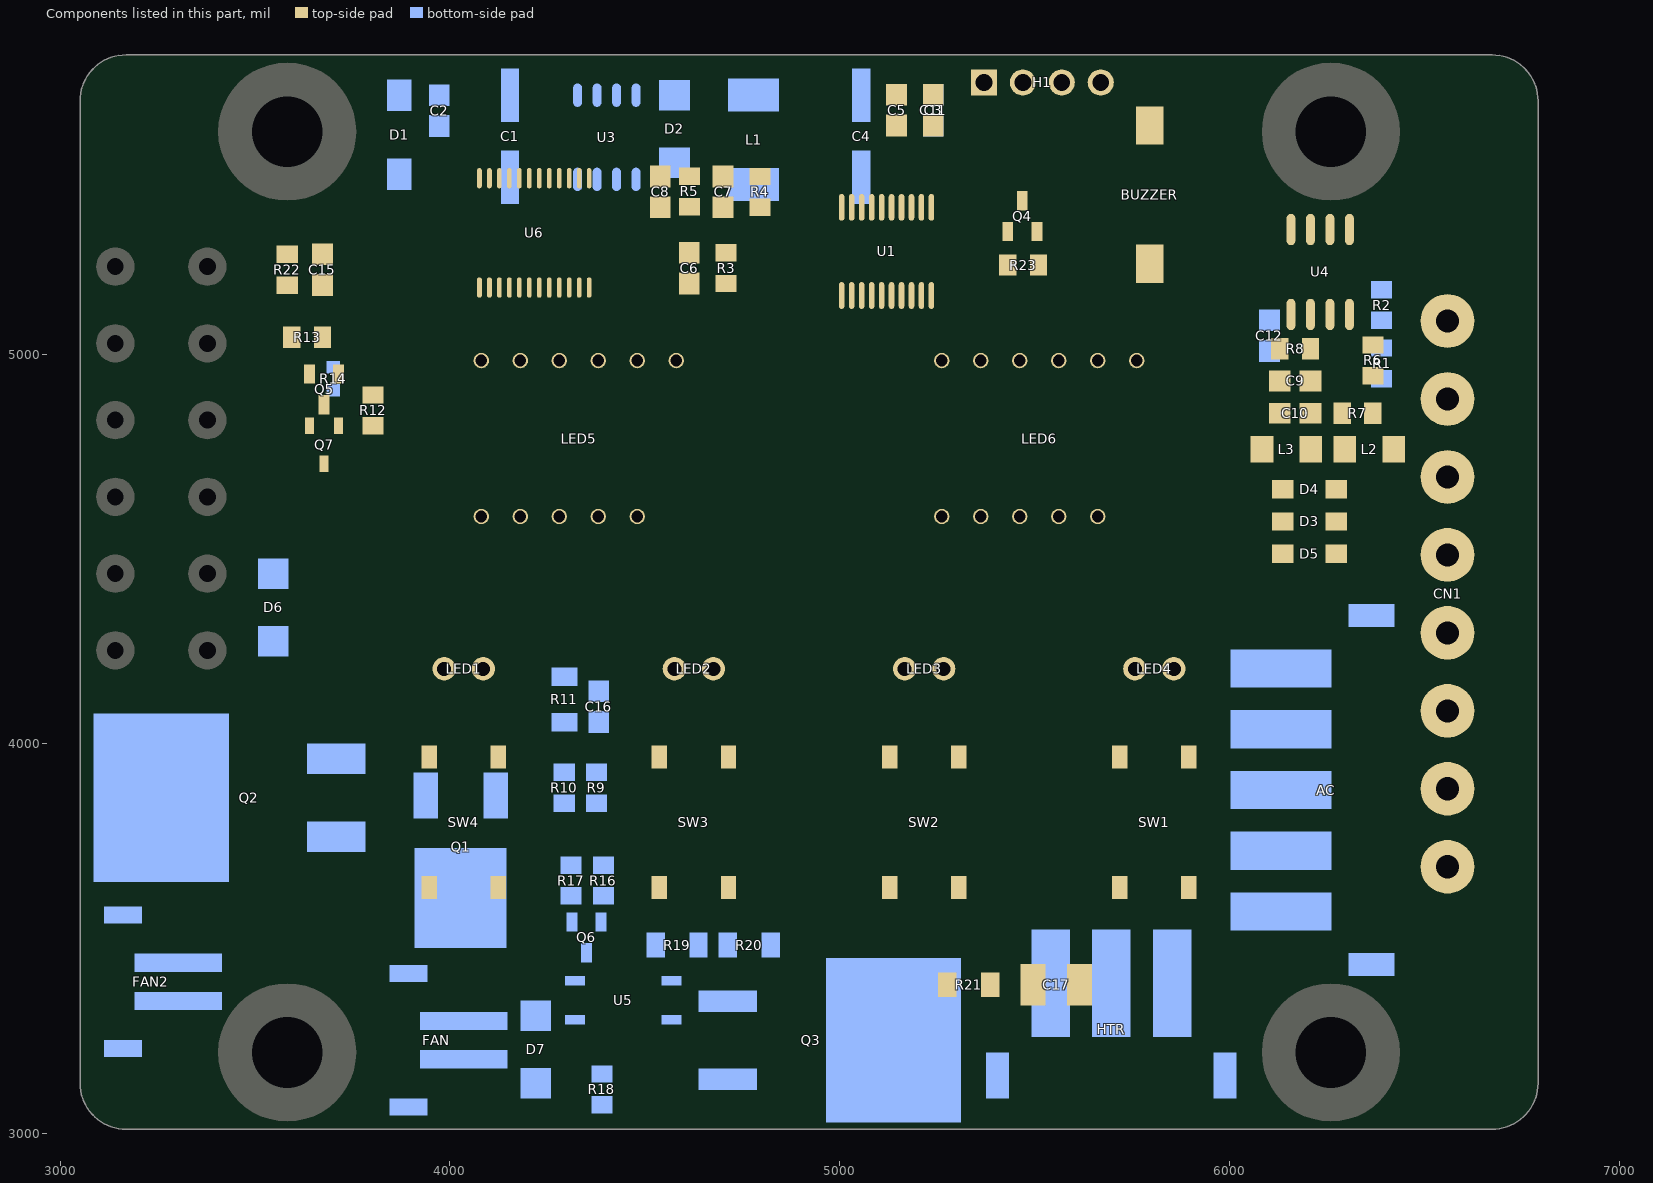
[diagram p0: the components of this part, seen from the top]
# Altium PCB MISC84275.PcbDoc (part 3 of 3)
Units mil, origin at the board's own origin, x right, y up, seen from the top; angles counter-clockwise.
Board outline 3740.1 x 2755.9 mil, 2 copper layers (Top Layer, Bottom Layer), stack 62.2 mil thick; 76 components, 62 nets, 275 pads, 150 vias.

## Polygon pours and split planes (outlines as drawn)
PL on Bottom Layer (solid, remove dead copper, pour order 62): 3093,4346.6 3566.8,4346.6 3592.5,4320.9 3592.5,3655.5 3570.9,3633.9 3090.6,3633.9 3070.9,3653.5 3070.9,4324.5
VCC on Top Layer (solid, remove dead copper, pour order 48): 3255.9,3665.4 3256.4,3665.4 3256.4,3664.9
N on Bottom Layer (solid, remove dead copper, pour order 72): 5992.1,3803.1 5992.1,3944.9 6007.9,3960.6 6763.8,3960.6 6773.6,3950.8 6773.6,3805.1 6763.8,3795.3 6000,3795.3
L on Bottom Layer (solid, remove dead copper, pour order 74): 6755.9,3748 6779.5,3724.4 6779.5,3039.4 6767.7,3027.6 6480.3,3027.6 6464.6,3043.3 6464.6,3378 6440.9,3401.6 6161.4,3401.6 6047.2,3287.4 6047.2,3271.7 6023.6,3248 5779.5,3248 5767.7,3259.8 5767.7,3519.7 5775.6,3527.6 5980.3,3527.6 5992.1,3539.4 5992.1,3637.8 6007.9,3653.5 6303.1,3653.5 6397.6,3748
HTR1 on Bottom Layer (solid, remove dead copper, pour order 76): 5318.9,3023.6 4899.1,3023.6 4889.8,3032.9 4889.8,3519.7 4901.6,3531.5 5602.4,3531.5 5606.3,3527.6 5606.3,3252 5590.6,3236.2 5350.4,3236.2 5330.7,3216.5 5330.7,3035.4
N on Bottom Layer (solid, remove dead copper, pour order 78): 5370.1,3039.4 5370.1,3203.5 5384.3,3217.8 6040.2,3217.8 6048.6,3209.4 6048.6,3032.9 6039.4,3023.6 5385.8,3023.6
N on Bottom Layer (solid, remove dead copper, pour order 80): 4626,3023.6 4606.3,3043.3 4606.3,3240.2 4618.1,3252 4831.9,3252 4846.5,3237.4 4846.5,3039.4 4830.7,3023.6
N on Top Layer (solid, remove dead copper, pour order 52): 4626,3023.6 4606.3,3043.3 4606.3,3263.8 4626,3283.5 5551.2,3283.5 5574.8,3307.1 5574.8,3494.5 5606.3,3526 5982.7,3526 6003.9,3547.2 6003.9,3956.7 6023.6,3976.4 6752,3976.4 6775.6,3952.8 6775.6,3803.1 6763.8,3791.3 6307.1,3791.3 6259.8,3744.1 6259.8,3535.4 6019.7,3295.3 6019.7,3055.1 5988.2,3023.6
L on Top Layer (solid, remove dead copper, pour order 56): 6397.6,3748 6755.9,3748 6779.5,3724.4 6779.5,3035.4 6771.7,3027.6 6507.9,3027.6 6488.2,3047.2 6488.2,3385.8 6397.6,3476.4
VCC on Bottom Layer (solid, remove dead copper, pour order 82): 3089.4,3589.8 3343.3,3589.8 3358.3,3574.8 3358.3,3539.4 3342.5,3523.6 3177.2,3523.6 3165.4,3511.8 3165.4,3393.7 3177.2,3381.9 3744.4,3381.9 3802.6,3440.2 3965.4,3440.2 3972.4,3433.1 3972.4,3385.8 3956.7,3370.1 3917.3,3370.1 3893.7,3346.5 3893.7,3244.1 3917.3,3220.5 4271.7,3220.5 4283.5,3208.7 4283.5,3029.5 4274.6,3020.5 3063,3020.5 3063,3563.3
FAN1 on Bottom Layer (solid, remove dead copper, pour order 84): 3932.5,3240.6 3913.4,3259.7 3913.4,3330.7 3937,3354.3 3964.6,3354.3 3989.4,3379.1 3989.4,3440.2 3972.8,3456.7 3795.3,3456.7 3740.2,3401.6 3196.9,3401.6 3185,3413.4 3185,3484.3 3203.4,3502.6 3383.1,3502.6 3443.5,3563 3803.1,3563 3838.7,3598.5 3838.7,3720.5 3850.5,3732.3 4192.9,3732.3 4263.8,3661.4 4263.8,3248 4256.3,3240.6
VCC on Top Layer (solid, remove dead copper, pour order 58): 3063,4732.3 3455.1,4732.3 3455.1,3575.9 3474.8,3556.3 4077.6,3556.3 4250.5,3383.3 4250.5,3030.1 4240.2,3019.7 3078.7,3019.7 3063,3035.4
GND1 on Bottom Layer (solid, remove dead copper, pour order 86): 3043.3,3003.9 3035.4,3011.8 3035.4,4881.9 3086.6,4933.1 3917.3,4933.1 3965.7,4884.7 3965.7,4617 4236.6,4346.1 5523.6,4346.1 5565.4,4304.3 5565.4,3622 5541.8,3598.4 4460.6,3598.4 4437,3574.8 4437,3027.6 4413.4,3003.9
GND1 on Top Layer (solid, remove dead copper, pour order 68): 4401.2,3000 3039.4,3000 3039.4,4940.9 3055.1,4956.7 3873.3,4956.7 3948.8,4881.1 3948.8,4629.9 4094.5,4484.3 4379.9,4484.3 4464.6,4399.6 4464.6,3599.1 4437,3571.5 4437,3035.8
GND on Bottom Layer (solid, remove dead copper, pour order 88): 3035.4,5791.3 6759.8,5791.3 6834.6,5716.5 6834.6,4511.8 6752,4429.1 6003.9,4429.1 5956.7,4476.4 5956.7,4921.3 5854.3,5023.6 3039.4,5023.6 3000,5063 3000,5755.9
GND on Top Layer (solid, remove dead copper, pour order 70): 3036.3,5773.6 6734.3,5773.6 6811,5696.9 6811,4492.1 6752,4433.1 6000,4433.1 5952.8,4480.3 5952.8,4925.2 5854.3,5023.6 3039.4,5023.6 3030.7,5032.3 3030.7,5768

## Keep-outs
Board Outline Layer:
  region: 5956.7,3980.3 ccw(c5956.7,3960.6) 5937,3960.6 5937,3606.3 ccw(c5956.7,3606.3) 5956.7,3586.6 ccw(c5956.7,3606.3) 5976.4,3606.3 5976.4,3960.6 ccw(c5956.7,3960.6) 5956.7,3980.3
  region: 5956.7,3980.3 ccw(c5956.7,3960.6) 5937,3960.6 5937,3606.3 ccw(c5956.7,3606.3) 5956.7,3586.6 ccw(c5956.7,3606.3) 5976.4,3606.3 5976.4,3960.6 ccw(c5956.7,3960.6) 5956.7,3980.3
  region: 5413.4,3563 ccw(c5433.1,3563) 5433.1,3543.3 5862.2,3543.3 ccw(c5862.2,3563) 5881.9,3563 ccw(c5862.2,3563) 5862.2,3582.7 5433.1,3582.7 ccw(c5433.1,3563) 5413.4,3563
  region: 5413.4,3563 ccw(c5433.1,3563) 5433.1,3543.3 5862.2,3543.3 ccw(c5862.2,3563) 5881.9,3563 ccw(c5862.2,3563) 5862.2,3582.7 5433.1,3582.7 ccw(c5433.1,3563) 5413.4,3563
  region: 4901.6,3563 ccw(c4921.3,3563) 4921.3,3543.3 5307.1,3543.3 ccw(c5307.1,3563) 5326.8,3563 ccw(c5307.1,3563) 5307.1,3582.7 4921.3,3582.7 ccw(c4921.3,3563) 4901.6,3563
  region: 4901.6,3563 ccw(c4921.3,3563) 4921.3,3543.3 5307.1,3543.3 ccw(c5307.1,3563) 5326.8,3563 ccw(c5307.1,3563) 5307.1,3582.7 4921.3,3582.7 ccw(c4921.3,3563) 4901.6,3563
  region: 4444.9,3563 ccw(c4464.6,3563) 4464.6,3543.3 4787.4,3543.3 ccw(c4787.4,3563) 4807.1,3563 ccw(c4787.4,3563) 4787.4,3582.7 4464.6,3582.7 ccw(c4464.6,3563) 4444.9,3563
  region: 4444.9,3563 ccw(c4464.6,3563) 4464.6,3543.3 4787.4,3543.3 ccw(c4787.4,3563) 4807.1,3563 ccw(c4787.4,3563) 4787.4,3582.7 4464.6,3582.7 ccw(c4464.6,3563) 4444.9,3563
  region: 4464.6,3464.6 ccw(c4464.6,3444.9) 4444.9,3444.9 4444.9,3082.7 ccw(c4464.6,3082.7) 4464.6,3063 ccw(c4464.6,3082.7) 4484.3,3082.7 4484.3,3444.9 ccw(c4464.6,3444.9) 4464.6,3464.6
  region: 4464.6,3464.6 ccw(c4464.6,3444.9) 4444.9,3444.9 4444.9,3082.7 ccw(c4464.6,3082.7) 4464.6,3063 ccw(c4464.6,3082.7) 4484.3,3082.7 4484.3,3444.9 ccw(c4464.6,3444.9) 4464.6,3464.6
  region: 6015.7,4385.4 ccw(c6035.4,4385.4) 6035.4,4365.8 6622,4365.8 ccw(c6622,4385.4) 6641.7,4385.4 ccw(c6622,4385.4) 6622,4405.1 6035.4,4405.1 ccw(c6035.4,4385.4) 6015.7,4385.4
  region: 6015.7,4385.4 ccw(c6035.4,4385.4) 6035.4,4365.8 6622,4365.8 ccw(c6622,4385.4) 6641.7,4385.4 ccw(c6622,4385.4) 6622,4405.1 6035.4,4405.1 ccw(c6035.4,4385.4) 6015.7,4385.4
  region: 5956.7,4354.3 ccw(c5956.7,4334.6) 5937,4334.6 5937,4059.1 ccw(c5956.7,4059.1) 5956.7,4039.4 ccw(c5956.7,4059.1) 5976.4,4059.1 5976.4,4334.6 ccw(c5956.7,4334.6) 5956.7,4354.3
  region: 5956.7,4354.3 ccw(c5956.7,4334.6) 5937,4334.6 5937,4059.1 ccw(c5956.7,4059.1) 5956.7,4039.4 ccw(c5956.7,4059.1) 5976.4,4059.1 5976.4,4334.6 ccw(c5956.7,4334.6) 5956.7,4354.3
  lines w0.1: 6035.4,4365.7 cw(c6035.4,4385.4) 6015.7,4385.4 ; 6622,4365.7 ccw(c6622,4385.4) 6641.7,4385.4 ; 4444.9,3082.7 4444.9,3444.9 ; 4444.9,3082.7 4444.9,3082.7 ; 4444.9,3082.7 ccw(c4464.6,3082.7) 4464.6,3063 ; 4444.9,3444.9 cw(c4464.6,3444.9) 4464.6,3464.6 ; 4444.9,3444.9 4444.9,3444.9 ; 4444.9,3563 ccw(c4464.6,3563) 4464.6,3543.3 ; 4444.9,3563 cw(c4464.6,3563) 4464.6,3582.7 ; 4444.9,3563 4444.9,3563 ; 4444.9,3563 4444.9,3563 ; 4464.6,3063 4464.6,3063 ; 4464.6,3063 4464.6,3063 ; 4464.6,3063 4464.6,3063 ; 4464.6,3063 ccw(c4464.6,3082.7) 4484.3,3082.7 ; 4464.6,3464.6 cw(c4464.6,3444.9) 4484.3,3444.9 ; 4464.6,3464.6 4464.6,3464.6 ; 4464.6,3464.6 4464.6,3464.6 ; 4464.6,3543.3 4464.6,3543.3 ; 4464.6,3543.3 4787.4,3543.3 ; 4464.6,3582.7 4787.4,3582.7 ; 4464.6,3582.7 4464.6,3582.7 ; 4484.3,3082.7 4484.3,3082.7 ; 4484.3,3082.7 4484.3,3444.9 ; 4484.3,3444.9 4484.3,3444.9 ; 4787.4,3543.3 4787.4,3543.3 ; 4787.4,3543.3 ccw(c4787.4,3563) 4807.1,3563 ; 4787.4,3582.7 cw(c4787.4,3563) 4807.1,3563 ; 4787.4,3582.7 4787.4,3582.7 ; 4807.1,3563 4807.1,3563 ; 4807.1,3563 4807.1,3563 ; 4807.1,3563 4807.1,3563 ; 4901.6,3563 ccw(c4921.3,3563) 4921.3,3543.3 5307.1,3543.3 ccw(c5307.1,3563) 5326.8,3563 ; 4901.6,3563 cw(c4921.3,3563) 4921.3,3582.7 5307.1,3582.7 cw(c5307.1,3563) 5326.8,3563 ; 4901.6,3563 4901.6,3563 ; 5326.8,3563 5326.8,3563 ; 5413.4,3563 ccw(c5433.1,3563) 5433.1,3543.3 ; 5413.4,3563 cw(c5433.1,3563) 5433.1,3582.7 ; 5413.4,3563 5413.4,3563 ; 5413.4,3563 5413.4,3563 ; 5433.1,3543.3 5433.1,3543.3 ; 5433.1,3543.3 5862.2,3543.3 ; 5433.1,3582.7 5862.2,3582.7 ; 5433.1,3582.7 5433.1,3582.7 ; 5862.2,3543.3 5862.2,3543.3 ; 5862.2,3543.3 ccw(c5862.2,3563) 5881.9,3563 ; 5862.2,3582.7 cw(c5862.2,3563) 5881.9,3563 ; 5862.2,3582.7 5862.2,3582.7 ; 5881.9,3563 5881.9,3563 ; 5881.9,3563 5881.9,3563 ; 5881.9,3563 5881.9,3563 ; 5956.7,3586.6 cw(c5956.7,3606.3) 5937,3606.3 5937,3960.6 cw(c5956.7,3960.6) 5956.7,3980.3 ; 5956.7,3586.6 5956.7,3586.6 ; 5956.7,3586.6 5956.7,3586.6 ; 5956.7,3586.6 5956.7,3586.6 ; 5956.7,3586.6 ccw(c5956.7,3606.3) 5976.4,3606.3 ; 5956.7,3980.3 cw(c5956.7,3960.6) 5976.4,3960.6 ; 5956.7,3980.3 5956.7,3980.3 ; 5956.7,3980.3 5956.7,3980.3 ; 5956.7,4039.4 cw(c5956.7,4059.1) 5937,4059.1 5937,4334.6 cw(c5956.7,4334.6) 5956.7,4354.3 ; 5956.7,4039.4 5956.7,4039.4 ; 5956.7,4039.4 ccw(c5956.7,4059.1) 5976.4,4059.1 5976.4,4334.6 ccw(c5956.7,4334.6) 5956.7,4354.3 ; 5956.7,4354.3 5956.7,4354.3 ; 5976.4,3606.3 5976.4,3606.3 ; 5976.4,3606.3 5976.4,3960.6 ; 5976.4,3960.6 5976.4,3960.6 ; 6015.7,4385.4 cw(c6035.4,4385.4) 6035.4,4405.1 ; 6015.7,4385.4 6015.7,4385.4 ; 6015.7,4385.4 6015.7,4385.4 ; 6035.4,4365.8 6035.4,4365.8 ; 6035.4,4365.8 6622,4365.8 ; 6035.4,4405.1 6622,4405.1 ; 6035.4,4405.1 6035.4,4405.1 ; 6622,4365.8 6622,4365.8 ; 6622,4405.1 cw(c6622,4385.4) 6641.7,4385.4 ; 6622,4405.1 6622,4405.1 ; 6641.7,4385.4 6641.7,4385.4 ; 6641.7,4385.4 6641.7,4385.4 ; 6641.7,4385.4 6641.7,4385.4
  lines w10: 6673.2,3011.8 3169.3,3011.8 cw(c3169.3,3129.9) 3051.2,3129.9 3051.2,5649.6 cw(c3169.3,5649.6) 3169.3,5767.7 6673.2,5767.7 ; 6673.2,3011.8 6673.2,3011.8 ; 6673.2,3011.8 ccw(c6673.2,3129.9) 6791.3,3129.9 ; 6673.2,5767.7 cw(c6673.2,5649.6) 6791.3,5649.6 ; 6673.2,5767.7 6673.2,5767.7 ; 6791.3,3129.9 6791.3,3129.9 ; 6791.3,3129.9 6791.3,5649.6 ; 6791.3,5649.6 6791.3,5649.6

## Silkscreen, mask and mechanical layers (free items; w line width, h text height)
Top Silkscreen Layer:
  lines w3.9: 3474.4,4141.4 3474.4,5381.9 3061,5381.9 3061,4141.7 3474.4,4141.7
  text "ENMG 26E26" at 4161.4,5626 h120
  text "5V" at 3259.8,5248 h49.2 r270
  text "AD" at 3259.8,5051.2 h49.2 r270
Bottom Silkscreen Layer:
  text "5V" at 3496.1,5192.9 h49.2 r270
  text "AD" at 3551.2,5055.1 h49.2 r90
  text "GND" at 3551.2,4874 h49.2 r90
  text "VCC" at 3551.2,4677.2 h49.2 r90
  text "VCC" at 3708.7,4484.3 h49.2 r90
  text "TEC" at 3708.7,4287.4 h49.2 r90
Top Solder Mask Layer:
  region: 4626,3023.6 4606.3,3043.3 4606.3,3263.8 4626,3283.5 5637.8,3283.5 5661.4,3307.1 5661.4,3490.6 5696.8,3526 5982.7,3526 6003.9,3547.2 6003.9,3956.7 6023.6,3976.4 6752,3976.4 6775.6,3952.8 6775.6,3803.1 6763.8,3791.3 6307.1,3791.3 6259.8,3744.1 6259.8,3535.4 6019.7,3295.3 6019.7,3055.1 5988.2,3023.6
  region: 6397.6,3748 6755.9,3748 6779.5,3724.4 6779.5,3035.4 6771.7,3027.6 6507.9,3027.6 6488.2,3047.2 6488.2,3385.8 6397.6,3476.4
  region: 4241.1,3030.8 3785.5,3030.8 3785.5,3332.6 3708.7,3409.4 3417.3,3409.4 3374,3366.1 3374,3059.1 3342.5,3027.6 3070.9,3027.6 3066.9,3023.6 3066.9,4051.2 3118.1,4102.4 3204.7,4102.4 3228.3,4126 3228.3,4334.6 3200.8,4362.2 3098.4,4362.2 3074.8,4385.8 3074.8,4700.8 3094.5,4720.5 3421.3,4720.5 3440.9,4700.8 3440.9,4389.8 3413.4,4362.2 3311,4362.2 3283.5,4334.6 3283.5,4126 3307.1,4102.4 3391.6,4102.4 3442.8,4051.1 3442.8,3565.1 3468.5,3539.4 4071.8,3539.4 4241.1,3370.1
Bottom Solder Mask Layer:
  lines w31.5: 4117.5,3960.2 4117.5,3987.6 4186.2,4056.3 4217.7,4056.3
  lines w39.4: 3102.4,4133.9 3533.1,4133.9 ; 3385.8,4736.2 3799.2,4736.2 3854.3,4681.1 3854.3,3803.1 3830.7,3779.5 ; 3452.8,3444.9 3511.8,3503.9 3826.8,3503.9 ; 3602.4,4645.7 3657.5,4590.6 3657.5,4539.4 ; 3755.9,4114.2 3755.9,4618.1 ; 3936.3,4449.6 4177.2,4208.7 4204.7,4208.7 ; 4019.7,4468.5 4196.9,4291.3 4370.1,4291.3 ; 4026.1,3395 4130.9,3395 ; 4192.9,3299.2 4192.9,3440.9 ; 4192.9,3688.7 4192.9,3440.9 ; 4952.8,3488.2 5448.8,3488.2 ; 5330.7,3295.3 5452.8,3295.3 ; 5330.7,3359.3 5453,3359.3 ; 5330.7,3421.3 5452.8,3421.3 ; 5440.9,3059.1 5956.7,3059.1 ; 5941.4,3355.1 5992.5,3406.3 6104.7,3406.3 ; 5956.7,3283.5 6000,3326.8 6043.3,3326.8 ; 5956.7,3444.9 5988.2,3476.4 6248.8,3475.7 ; 6311,3527.6 6366.1,3527.6 6448.8,3610.2 ; 6311,3606.3 6362.2,3606.3 6448.8,3692.9 ; 6433.1,3500 6728.3,3500 ; 6523.6,3570.9 6716.5,3570.9 ; 6539.4,3059.1 6539.4,3430 ; 6618.1,3059.1 6618.1,3429.1 ; 6689,3066.9 6689,3433.1 ; 4192.9,3440.9 4192.9,3440.9
Mechanical Layer:
  lines w0.1: 6035.4,4365.7 cw(c6035.4,4385.4) 6015.7,4385.4 ; 6622,4365.7 ccw(c6622,4385.4) 6641.7,4385.4 ; 4444.9,3082.7 4444.9,3444.9 ; 4444.9,3082.7 4444.9,3082.7 ; 4444.9,3082.7 ccw(c4464.6,3082.7) 4464.6,3063 ; 4444.9,3444.9 cw(c4464.6,3444.9) 4464.6,3464.6 ; 4444.9,3444.9 4444.9,3444.9 ; 4444.9,3563 ccw(c4464.6,3563) 4464.6,3543.3 ; 4444.9,3563 cw(c4464.6,3563) 4464.6,3582.7 ; 4444.9,3563 4444.9,3563 ; 4444.9,3563 4444.9,3563 ; 4464.6,3063 4464.6,3063 ; 4464.6,3063 4464.6,3063 ; 4464.6,3063 4464.6,3063 ; 4464.6,3063 ccw(c4464.6,3082.7) 4484.3,3082.7 ; 4464.6,3464.6 cw(c4464.6,3444.9) 4484.3,3444.9 ; 4464.6,3464.6 4464.6,3464.6 ; 4464.6,3464.6 4464.6,3464.6 ; 4464.6,3543.3 4464.6,3543.3 ; 4464.6,3543.3 4787.4,3543.3 ; 4464.6,3582.7 4787.4,3582.7 ; 4464.6,3582.7 4464.6,3582.7 ; 4484.3,3082.7 4484.3,3082.7 ; 4484.3,3082.7 4484.3,3444.9 ; 4484.3,3444.9 4484.3,3444.9 ; 4787.4,3543.3 4787.4,3543.3 ; 4787.4,3543.3 ccw(c4787.4,3563) 4807.1,3563 ; 4787.4,3582.7 cw(c4787.4,3563) 4807.1,3563 ; 4787.4,3582.7 4787.4,3582.7 ; 4807.1,3563 4807.1,3563 ; 4807.1,3563 4807.1,3563 ; 4807.1,3563 4807.1,3563 ; 4901.6,3563 ccw(c4921.3,3563) 4921.3,3543.3 5307.1,3543.3 ccw(c5307.1,3563) 5326.8,3563 ; 4901.6,3563 cw(c4921.3,3563) 4921.3,3582.7 5307.1,3582.7 cw(c5307.1,3563) 5326.8,3563 ; 4901.6,3563 4901.6,3563 ; 5326.8,3563 5326.8,3563 ; 5413.4,3563 ccw(c5433.1,3563) 5433.1,3543.3 ; 5413.4,3563 cw(c5433.1,3563) 5433.1,3582.7 ; 5413.4,3563 5413.4,3563 ; 5413.4,3563 5413.4,3563 ; 5433.1,3543.3 5433.1,3543.3 ; 5433.1,3543.3 5862.2,3543.3 ; 5433.1,3582.7 5862.2,3582.7 ; 5433.1,3582.7 5433.1,3582.7 ; 5862.2,3543.3 5862.2,3543.3 ; 5862.2,3543.3 ccw(c5862.2,3563) 5881.9,3563 ; 5862.2,3582.7 cw(c5862.2,3563) 5881.9,3563 ; 5862.2,3582.7 5862.2,3582.7 ; 5881.9,3563 5881.9,3563 ; 5881.9,3563 5881.9,3563 ; 5881.9,3563 5881.9,3563 ; 5956.7,3586.6 cw(c5956.7,3606.3) 5937,3606.3 5937,3960.6 cw(c5956.7,3960.6) 5956.7,3980.3 ; 5956.7,3586.6 5956.7,3586.6 ; 5956.7,3586.6 5956.7,3586.6 ; 5956.7,3586.6 5956.7,3586.6 ; 5956.7,3586.6 ccw(c5956.7,3606.3) 5976.4,3606.3 ; 5956.7,3980.3 cw(c5956.7,3960.6) 5976.4,3960.6 ; 5956.7,3980.3 5956.7,3980.3 ; 5956.7,3980.3 5956.7,3980.3 ; 5956.7,4039.4 cw(c5956.7,4059.1) 5937,4059.1 5937,4334.6 cw(c5956.7,4334.6) 5956.7,4354.3 ; 5956.7,4039.4 5956.7,4039.4 ; 5956.7,4039.4 ccw(c5956.7,4059.1) 5976.4,4059.1 5976.4,4334.6 ccw(c5956.7,4334.6) 5956.7,4354.3 ; 5956.7,4354.3 5956.7,4354.3 ; 5976.4,3606.3 5976.4,3606.3 ; 5976.4,3606.3 5976.4,3960.6 ; 5976.4,3960.6 5976.4,3960.6 ; 6015.7,4385.4 cw(c6035.4,4385.4) 6035.4,4405.1 ; 6015.7,4385.4 6015.7,4385.4 ; 6015.7,4385.4 6015.7,4385.4 ; 6035.4,4365.8 6035.4,4365.8 ; 6035.4,4365.8 6622,4365.8 ; 6035.4,4405.1 6622,4405.1 ; 6035.4,4405.1 6035.4,4405.1 ; 6622,4365.8 6622,4365.8 ; 6622,4405.1 cw(c6622,4385.4) 6641.7,4385.4 ; 6622,4405.1 6622,4405.1 ; 6641.7,4385.4 6641.7,4385.4 ; 6641.7,4385.4 6641.7,4385.4 ; 6641.7,4385.4 6641.7,4385.4